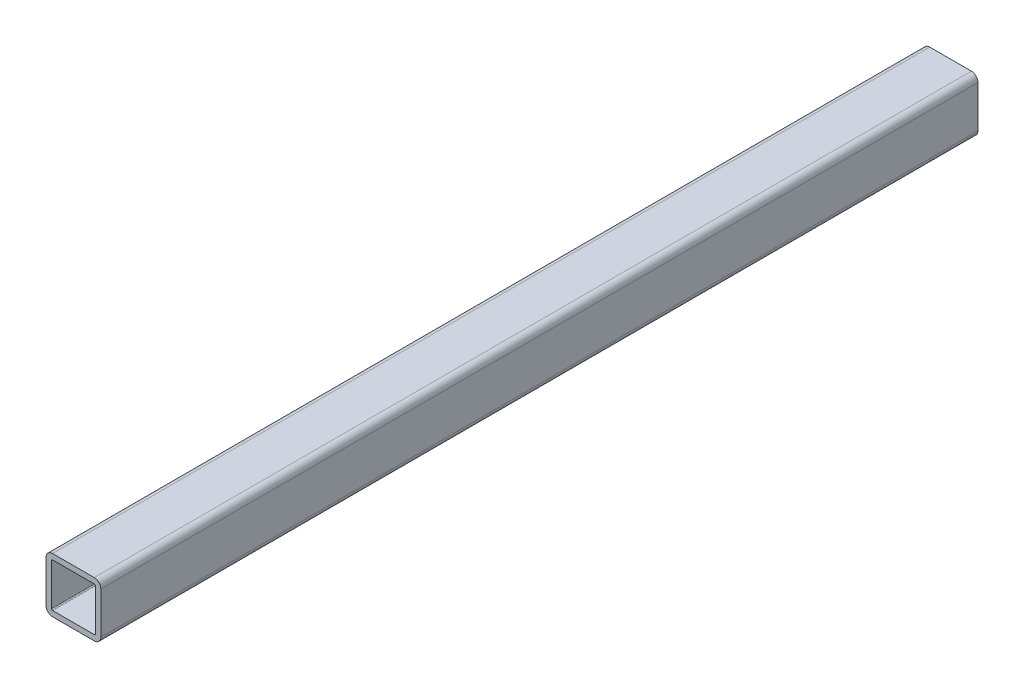
SolidWorks part; units mm, degrees
material "Q235B"
ref_plane "Front Plane" through (0, 0, 0) normal (0, 0, 1) x (1, 0, 0)
ref_plane "Top Plane" through (0, 0, 0) normal (0, 1, 0) x (1, 0, 0)
ref_plane "Right Plane" through (0, 0, 0) normal (1, 0, 0) x (0, 0, -1)
sketch "Sketch1" plane through (0, 0, 0) normal (0, 0, 1) x (1, 0, 0)
  line L0 (6, 45) -> (44, 45)
  line L1 (6, 0) -> (44, 0)
  line L2 (0, 6) -> (0, 44)
  line L3 (6, 50) -> (44, 50)
  line L4 (50, 6) -> (50, 44)
  line L5 (45, 6) -> (45, 44)
  line L6 (6, 5) -> (44, 5)
  line L7 (5, 6) -> (5, 44)
  arc A0 (6, 0) -> (0, 6) centre (6, 6) cw
  arc A1 (44, 0) -> (50, 6) centre (44, 6) ccw
  arc A2 (44, 50) -> (50, 44) centre (44, 44) cw
  arc A3 (0, 44) -> (6, 50) centre (6, 44) cw
  arc A4 (5, 44) -> (6, 45) centre (6, 44) cw
  arc A5 (44, 45) -> (45, 44) centre (44, 44) cw
  arc A6 (44, 5) -> (45, 6) centre (44, 6) ccw
  arc A7 (6, 5) -> (5, 6) centre (6, 6) cw
  point P7 (0, 0)
  point P12 (50, 50)
  point P15 (0, 50)
  dimension "D3" = 6
  dimension "D1" = 50
  dimension "D2" = 50
  dimension "D4" = 5
extrude "Boss-Extrude1" add sketch "Sketch1" along normal blind 800
